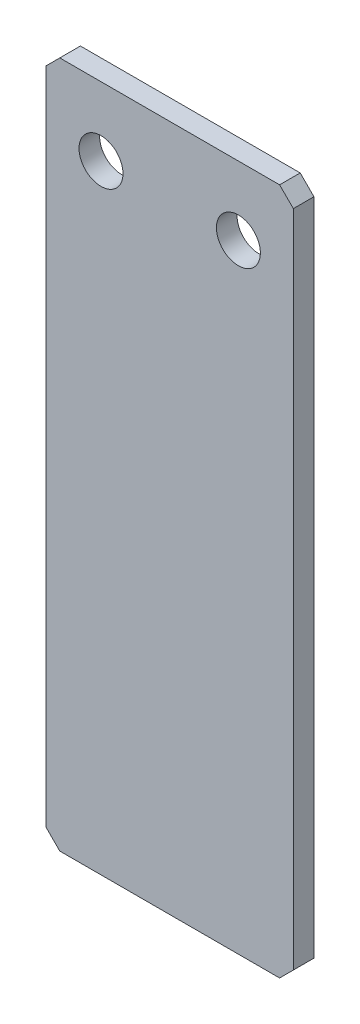
from build123d import *

# Parameters (mm, degrees)
SKETCH1_W                      = 18
SKETCH1_H                      = 50
BOSS_EXTRUDE1_DEPTH            = 1.5
F_3_2_3_2_DIAMETER_HOLE1_D     = 3.2
F_3_2_3_2_DIAMETER_HOLE1_DEPTH = 12
F_3_2_3_2_DIAMETER_HOLE1_TIP   = 0.96137699
CHAMFER1_SIZE                  = 1


with BuildPart() as part:
    # Sketch1 → Boss-Extrude1 (new body)
    with BuildSketch(Plane.XY):
        Rectangle(SKETCH1_W, SKETCH1_H)
    extrude(amount=BOSS_EXTRUDE1_DEPTH)

    # Ø3.2 (3.2) Diameter Hole1
    with Locations(Plane.XY.offset(1.5)):
        with Locations((-5, 20), (5, 20)):
            Hole(F_3_2_3_2_DIAMETER_HOLE1_D / 2, depth=F_3_2_3_2_DIAMETER_HOLE1_DEPTH)
            with Locations((0, 0, -(F_3_2_3_2_DIAMETER_HOLE1_DEPTH + F_3_2_3_2_DIAMETER_HOLE1_TIP / 2))):  # 118° drill point
                Cone(0, F_3_2_3_2_DIAMETER_HOLE1_D / 2, F_3_2_3_2_DIAMETER_HOLE1_TIP, mode=Mode.SUBTRACT)

    # Chamfer1
    chamfer1_edges = [part.edges().sort_by_distance(p)[0] for p in [
        (9, -25, 0.75),
        (-9, -25, 0.75),
        (-9, 25, 0.75),
        (9, 25, 0.75),
    ]]
    chamfer(chamfer1_edges, length=CHAMFER1_SIZE)


solid = part.part
